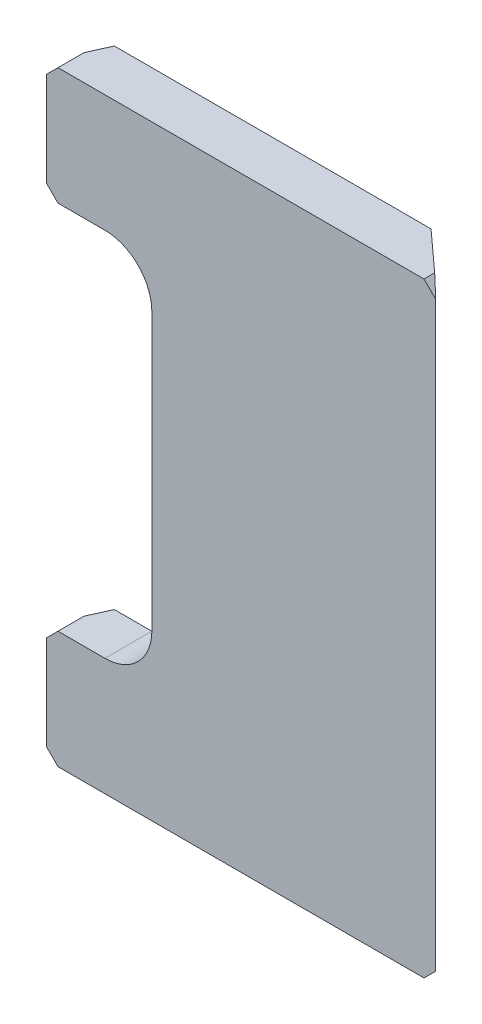
SolidWorks part; units mm, degrees
ref_plane "Front Plane" through (0, 0, 0) normal (0, 0, 1) x (1, 0, 0)
ref_plane "Top Plane" through (0, 0, 0) normal (0, 1, 0) x (1, 0, 0)
ref_plane "Right Plane" through (0, 0, 0) normal (1, 0, 0) x (0, 0, -1)
sketch "Sketch1" plane through (0, 0, 0) normal (0, 0, 1) x (1, 0, 0)
  line L0 (45, 188) -> (45, 70)
  line L1 (5, 0) -> (161, 0)
  line L2 (0, 5) -> (0, 45)
  line L3 (5, 258) -> (161, 258)
  line L4 (166, 5) -> (166, 253)
  line L5 (5, 208) -> (25, 208)
  line L6 (5, 50) -> (25, 50)
  line L7 (161, 0) -> (166, 5)
  line L8 (166, 253) -> (161, 258)
  line L9 (0, 253) -> (5, 258)
  line L10 (0, 5) -> (5, 0)
  line L11 (0, 45) -> (5, 50)
  line L12 (0, 253) -> (0, 213)
  line L13 (0, 213) -> (5, 208)
  arc A0 (25, 50) -> (45, 70) centre (25, 70) ccw
  arc A1 (25, 208) -> (45, 188) centre (25, 188) cw
  point P0 (0, 0)
  point P1 (166, 258)
  point P2 (0, 258)
  point P3 (166, 0)
  point P23 (0, 50)
  point P26 (0, 208)
  dimension "D6" = 20
  dimension "D7" = 20
  dimension "D1" = 258
  dimension "D2" = 166
  dimension "D3" = 121
  dimension "D4" = 50
  dimension "D5" = 50
  dimension "D8" = 5
  dimension "D9" = 45
  dimension "D10" = 5
  dimension "D11" = 45
  dimension "D12" = 5
  dimension "D13" = 45
  dimension "D14" = 5
  dimension "D15" = 45
  dimension "D16" = 5
  dimension "D17" = 45
  dimension "D18" = 5
  dimension "D19" = 45
extrude "Boss-Extrude1" add sketch "Sketch1" along normal blind 20
sketch "Sketch2" plane through (0, 0, 0) normal (0, -1, 0) x (1, 0, 0)
  line L0 (0, 20) -> (0, 0) construction
  line L1 (0, 20) -> (0, 0)
  line L2 (166, 20) -> (166, 0) construction
  line L3 (5, 0) -> (161, 0) construction
  line L4 (166, 20) -> (166, 0)
  line L5 (0, 0) -> (9, 0)
  line L6 (0, 20) -> (9, 0)
  line L7 (166, 20) -> (144, 0)
  line L8 (144, 0) -> (166, 0)
  dimension "D1" = 22
  dimension "D2" = 9
extrude "Cut-Extrude1" cut sketch "Sketch2" along direction (0, 1, 0) on the side against the normal through all
